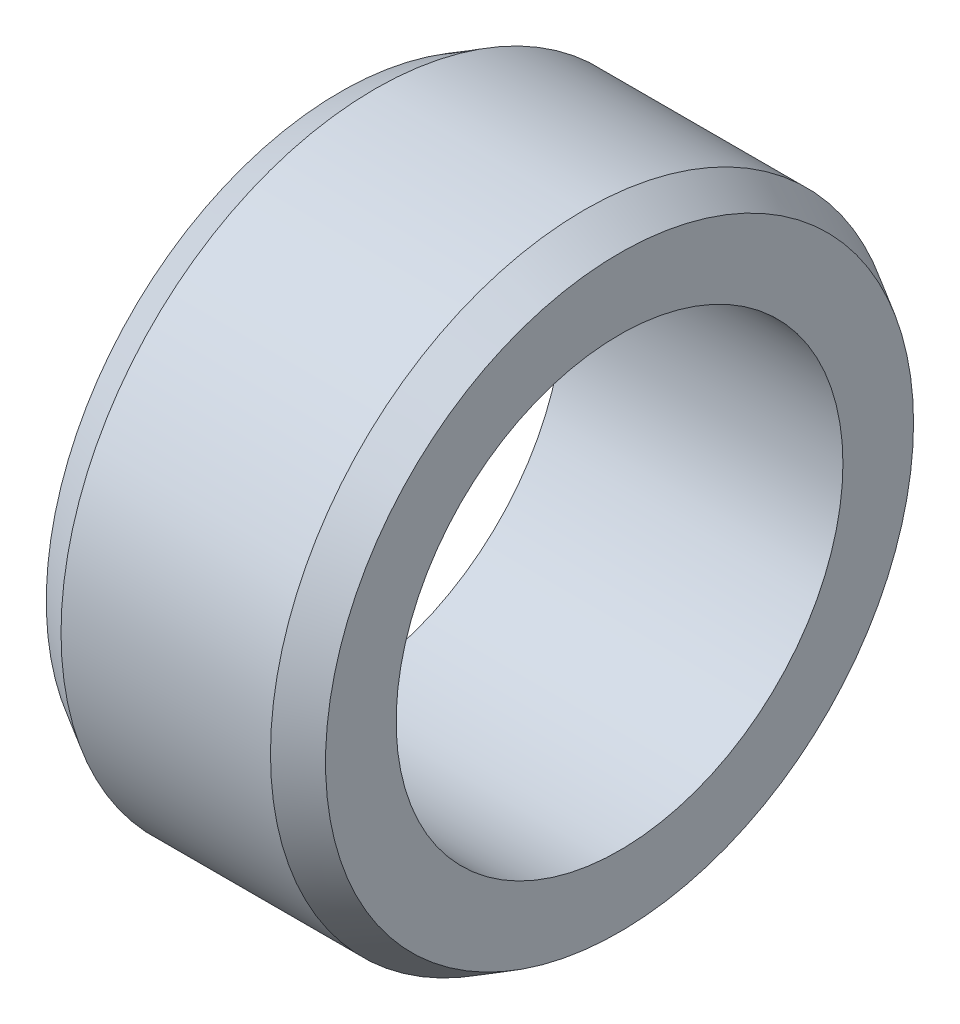
from build123d import *


with BuildPart() as part:
    # Sketch1 → Revolve1 (revolve)
    with BuildSketch(Plane.XY, mode=Mode.PRIVATE) as revolve1_sk:
        Polygon((0, 3.2), (4, 3.2), (4, 4.211324865), (3.5, 4.5), (0.5, 4.5), (0, 4.211324865), align=None)
    revolve(revolve1_sk.sketch.rotate(Axis((4, 0, 0), (-1, 0, 0)), 90), axis=Axis((4, 0, 0), (-1, 0, 0)))


solid = part.part
